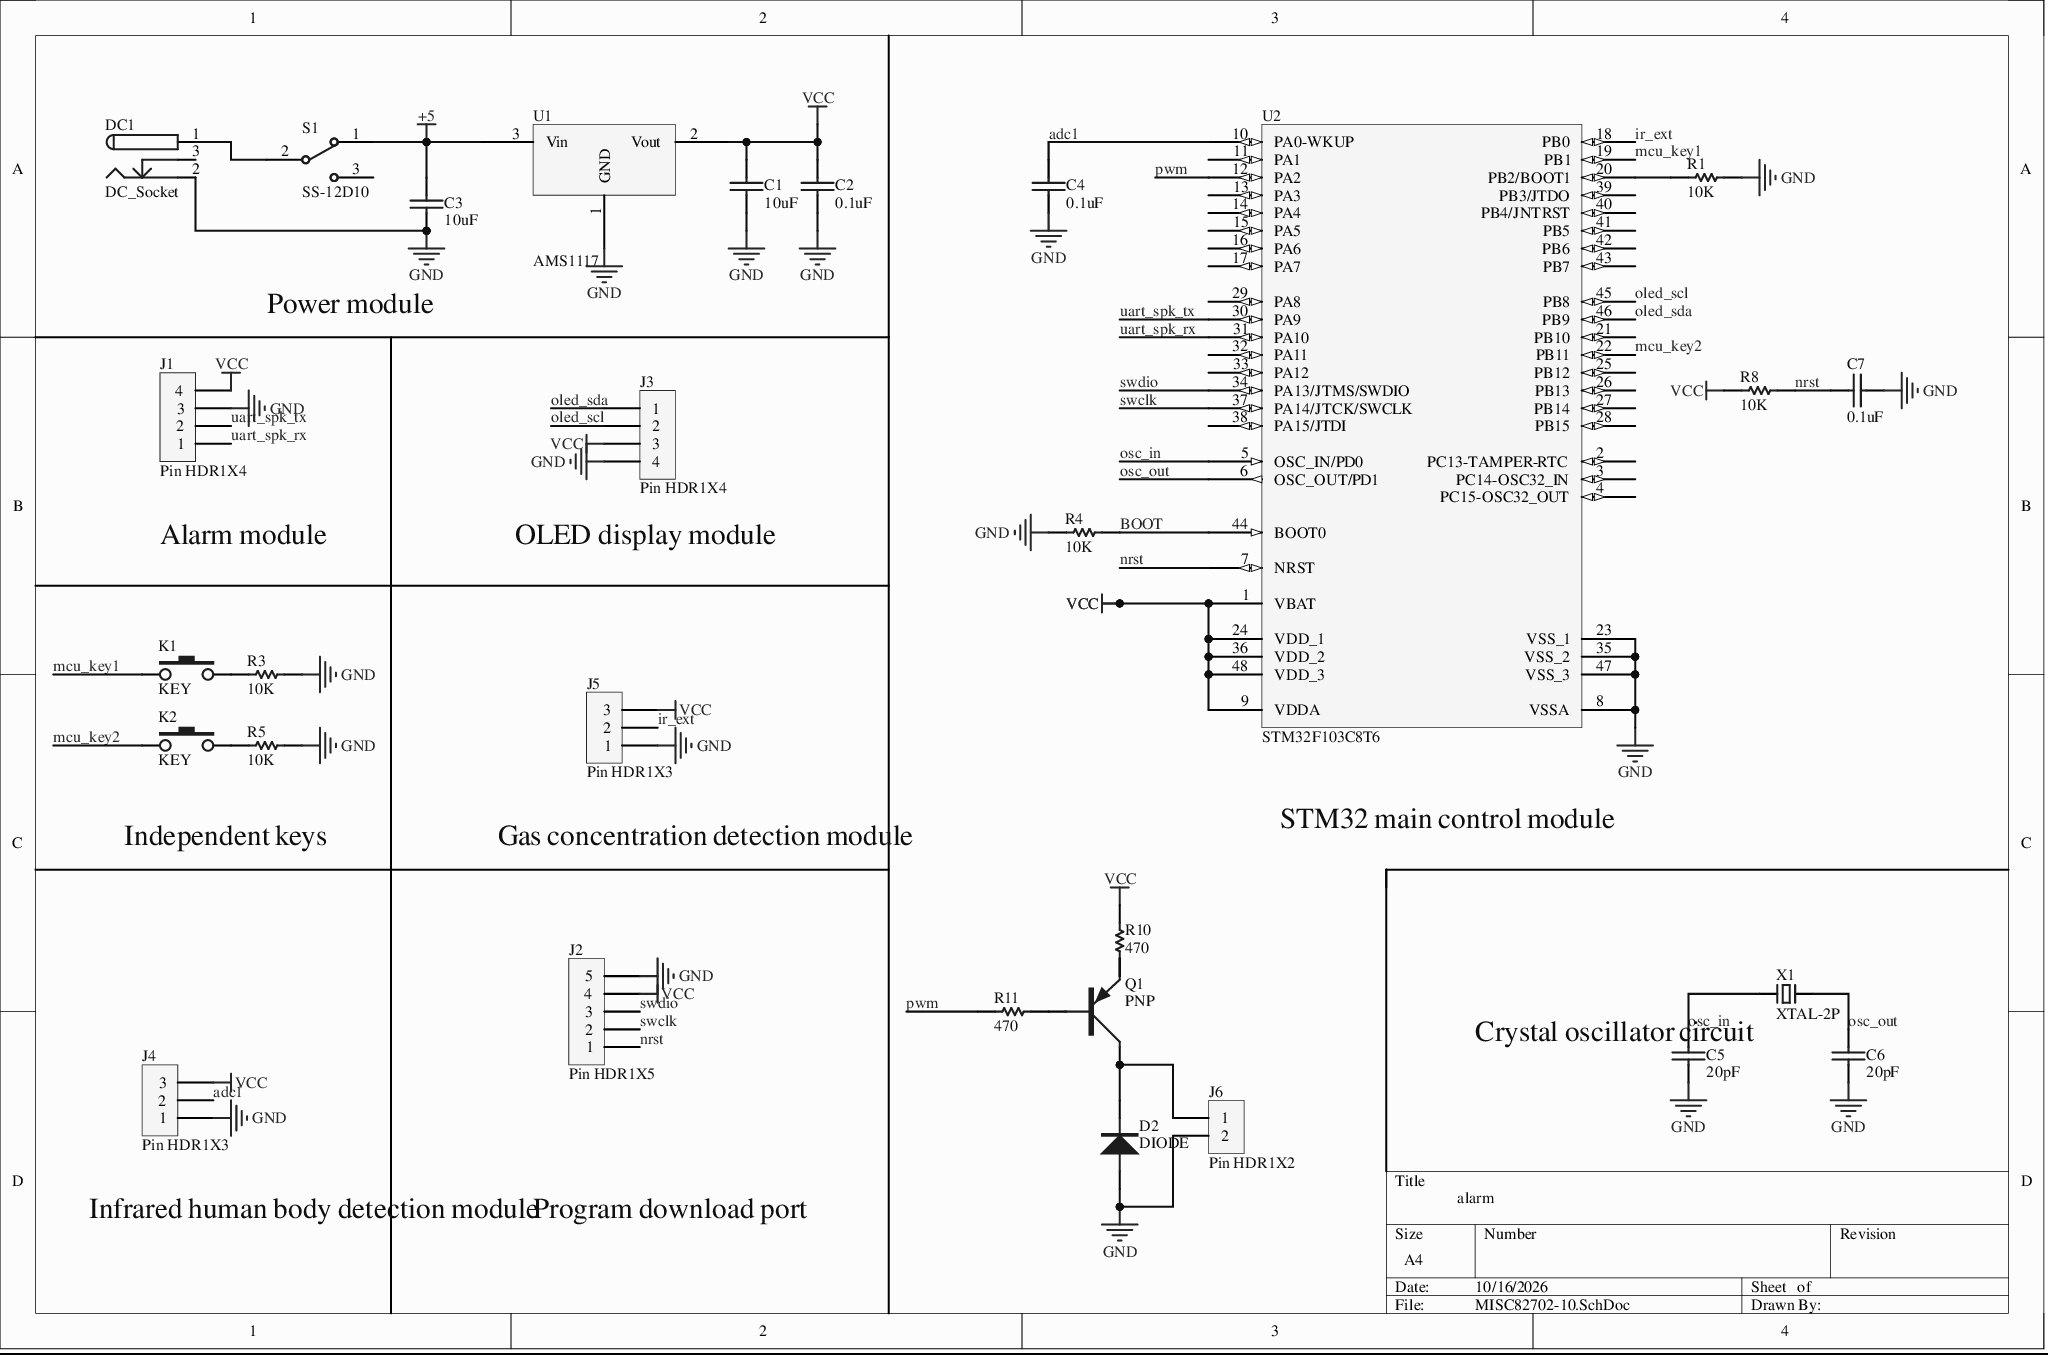
[diagram p0: MISC82702-10.SchDoc]
# Altium project MISC82702-6.PrjPCB
1 sheet, 29 parts. Net scope: global (net labels, ports and power ports of the same name join across sheets).
Board file: MISC82702.PcbDoc

## Sheet MISC82702-10.SchDoc
size A4

### Parts
C1  10uF  [0603C]
C2  0.1uF  [0603C]
C3  10uF  [0603C]
C4  0.1uF  [0603C]
C5  20pF  [0603C]
C6  20pF  [0603C]
C7  0.1uF  [0603C]
D2  DIODE  [SOD-123]
DC1  DC_Socket  [DC-002]
J1  Pin HDR1X4  [Pin HDR1X4/2.54mm-S]
J2  Pin HDR1X5  [Pin HDR1X5/2.54mm-S]
J3  Pin HDR1X4  [Pin HDR1X4/2.54mm-S]
J4  Pin HDR1X3  [Pin HDR1X3/2.54mm-S]
J5  Pin HDR1X3  [Pin HDR1X3/2.54mm-S]
J6  Pin HDR1X2  [Pin HDR1X2/2.54mm-S]
K1  KEY  [DIP-3X6X4.3]
K2  KEY  [DIP-3X6X4.3]
Q1  PNP  [SOT-23]
R1  10K  [0603R]
R3  10K  [0603R]
R4  10K  [0603R]
R5  10K  [0603R]
R8  10K  [0603R]
R10  470  [0603R]
R11  470  [0603R]
S1  SS-12D10  [SS-12D10]
U1  AMS1117  [SOT223]
U2  STM32F103C8T6  [LQFP48 7X7]
X1  XTAL-2P  [OSC HC-49S]

### Nets
+5: C3.2 S1.1 U1.3(Vin)
GND: C1.1 C2.1 C3.1 C4.1 C5.1 C6.1 C7.1 D2.A DC1.2 J1.3 J2.5 J3.4 J4.1 J5.1 J6.2 R1.1 R3.1 R4.2 R5.1 U1.1(GND) U2.8(VSSA) U2.23(VSS_1) U2.35(VSS_2) U2.47(VSS_3)
VCC: C1.2 C2.2 J1.4 J2.4 J3.3 J4.3 J5.3 R8.2 R10.1 U1.2(Vout) U2.1(VBAT) U2.9(VDDA) U2.24(VDD_1) U2.36(VDD_2) U2.48(VDD_3)
adc1: C4.2 J4.2 U2.10(PA0-WKUP)
BOOT: R4.1 U2.44(BOOT0)
ir_ext: J5.2 U2.18(PB0)
mcu_key1: K1.1 U2.19(PB1)
mcu_key2: K2.1 U2.22(PB11)
nrst: C7.2 J2.1 R8.1 U2.7(NRST)
oled_scl: J3.2 U2.45(PB8)
oled_sda: J3.1 U2.46(PB9)
osc_in: C5.2 U2.5(OSC_IN/PD0) X1.1
osc_out: C6.2 U2.6(OSC_OUT/PD1) X1.2
pwm: R11.1 U2.12(PA2)
swclk: J2.2 U2.37(PA14/JTCK/SWCLK)
swdio: J2.3 U2.34(PA13/JTMS/SWDIO)
uart_spk_rx: J1.1 U2.31(PA10)
uart_spk_tx: J1.2 U2.30(PA9)
NetD2_K: D2.K J6.1 Q1.C
NetDC1_1: DC1.1 S1.2
NetK1_3: K1.3 R3.2
NetK2_3: K2.3 R5.2
NetQ1_B: Q1.B R11.2
NetQ1_E: Q1.E R10.2
NetR1_2: R1.2 U2.20(PB2/BOOT1)

Not connected (* = marked no-connect by the designer): DC1 3; S1 3; U2 2(PC13-TAMPER-RTC) 3(PC14-OSC32_IN) 4(PC15-OSC32_OUT) 11(PA1) 13(PA3) 14(PA4) 15(PA5) 16(PA6) 17(PA7) 21(PB10) 25(PB12) 26(PB13) 27(PB14) 28(PB15) 29(PA8) 32(PA11) 33(PA12) 38(PA15/JTDI) 39(PB3/JTDO) 40(PB4/JNTRST) 41(PB5) 42(PB6) 43(PB7)

### Notes on the sheet
- Power module
- Alarm module
- (near J3) OLED display module
- Independent keys
- Gas concentration detection module
- STM32 main control module
- Crystal oscillator circuit
- alarm
- Infrared human body detection module
- Program download port

### Library data of the parts
C1-C7 = CAP: Non-polar capacitor
D2 = DIODE: General-purpose diode
Q1 = PNP: PNP transistor
R1 R3-R5 R8 R10 R11 = RES
U1 = AMS1117: Three-terminal voltage regulator
X1 = XTAL-2P: 2-pin passive crystal oscillator